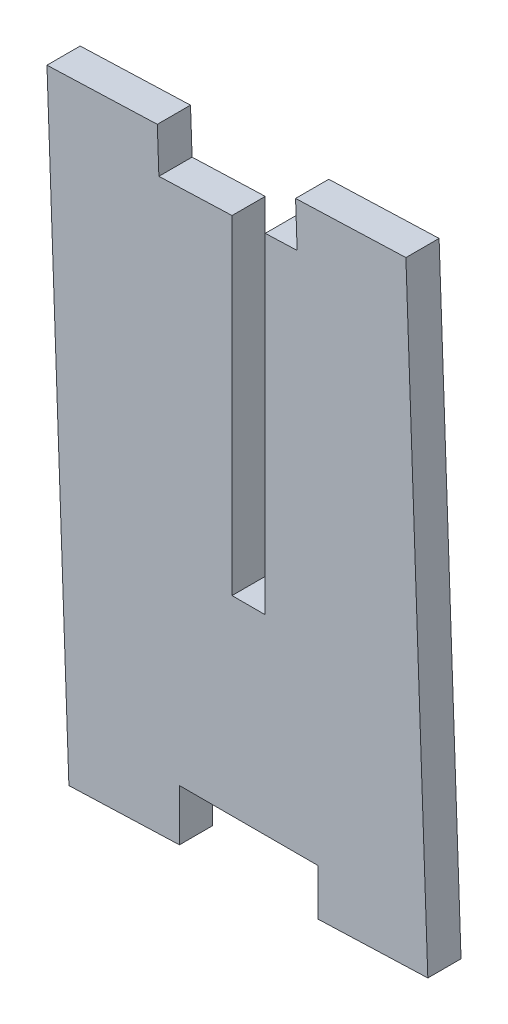
from build123d import *

# Parameters (mm, degrees)
BOSS_EXTRUDE1_DEPTH = 6
SKETCH2_W           = 6
SKETCH2_H           = 59.975118876
CUT_EXTRUDE1_DEPTH  = 6


with BuildPart() as part:
    # Sketch1 → Boss-Extrude1 (new body)
    with BuildSketch(Plane.XY):
        Polygon((106.551616656, -20.563894675), (102.587015051, 90.196105325), (122.52424687, 90.909749071), (122.810419801, 82.914869143), (147.794419574, 83.809159551), (147.508246643, 91.804039479), (167.445478462, 92.517683224), (171.410080068, -18.242316776), (151.529151094, -18.953945188), (151.529151094, -10.563897816), (126.528434018, -10.563897816), (126.528434018, -19.848833984), align=None)
    extrude(amount=BOSS_EXTRUDE1_DEPTH)

    # Sketch2 → Cut-Extrude1 (cut)
    with BuildSketch(Plane.XY.offset(6)):
        with Locations((139.028792556, 53.898004923)):
            Rectangle(SKETCH2_W, SKETCH2_H)
    extrude(amount=-CUT_EXTRUDE1_DEPTH, mode=Mode.SUBTRACT)


solid = part.part
